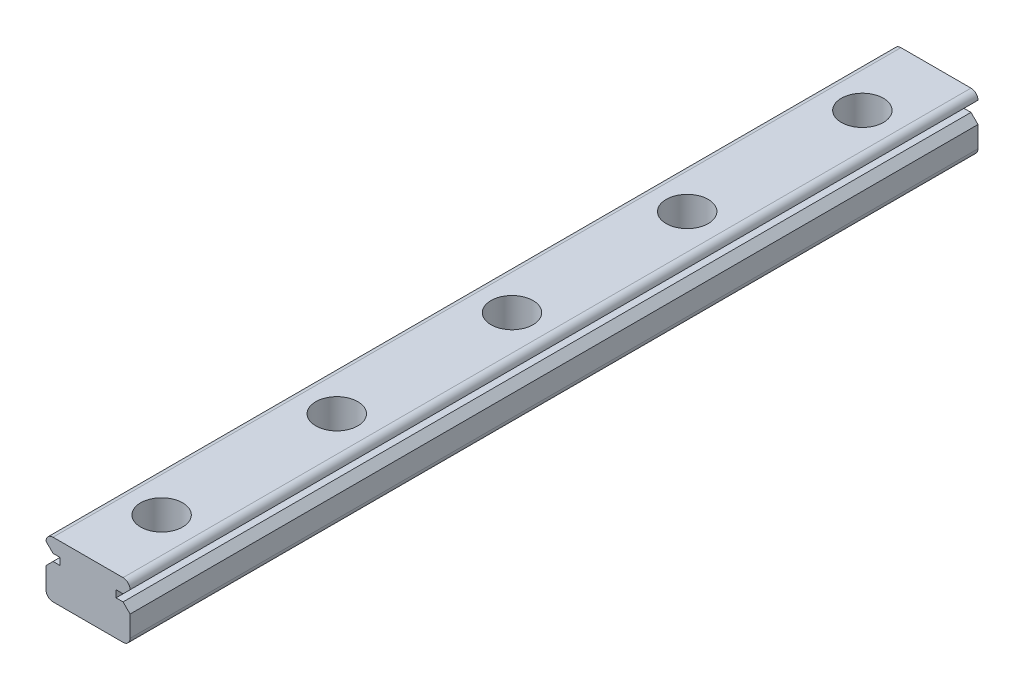
from build123d import *

# Parameters (mm, degrees)
BOSS_EXTRUDE1_DEPTH = 121
SKETCH2_R           = 3
CUT_EXTRUDE1_DEPTH  = 4.5
SKETCH3_R           = 1.75
CUT_EXTRUDE2_DEPTH  = 122.232215191


with BuildPart() as part:
    # Sketch1 → Boss-Extrude1 (new body)
    with BuildSketch(Plane.XY):
        with BuildLine():
            Line((-5, 4), (5, 4))
            ThreePointArc((5, 4), (5.707106781, 3.707106781), (6, 3))
            Line((6, 3), (5, 2))
            Line((5, 2), (4, 2))
            Line((4, 2), (4, 1))
            Line((4, 1), (5, 1))
            Line((5, 1), (6, 0))
            Line((6, 0), (6, -3))
            ThreePointArc((6, -3), (5.707106781, -3.707106781), (5, -4))
            Line((5, -4), (-5, -4))
            ThreePointArc((-5, -4), (-5.707106781, -3.707106781), (-6, -3))
            Line((-6, -3), (-6, 0))
            Line((-6, 0), (-5, 1))
            Line((-5, 1), (-4, 1))
            Line((-4, 1), (-4, 2))
            Line((-4, 2), (-5, 2))
            Line((-5, 2), (-6, 3))
            ThreePointArc((-6, 3), (-5.707106781, 3.707106781), (-5, 4))
        make_face()
    extrude(amount=BOSS_EXTRUDE1_DEPTH)

    # Sketch2 → Cut-Extrude1 (cut)
    with BuildSketch(Plane(origin=(0, 4, 0), x_dir=(1, 0, 0), z_dir=(0, 1, 0))):
        with Locations(Location((0, -10.5, 0), (0, 0, 270))):
            Circle(SKETCH2_R)
        with Locations(Location((0, -35.5, 0), (0, 0, 270))):
            Circle(SKETCH2_R)
        with Locations(Location((0, -60.5, 0), (0, 0, 270))):
            Circle(SKETCH2_R)
        with Locations(Location((0, -85.5, 0), (0, 0, 270))):
            Circle(SKETCH2_R)
        with Locations(Location((0, -110.5, 0), (0, 0, 270))):
            Circle(SKETCH2_R)
    extrude(amount=-CUT_EXTRUDE1_DEPTH, mode=Mode.SUBTRACT)

    # Sketch3 → Cut-Extrude2 (cut, through all)
    with BuildSketch(Plane(origin=(0, -0.5, 0), x_dir=(1, 0, 0), z_dir=(0, 1, 0))):
        with Locations(Location((0, -35.5, 0), (0, 0, 270))):
            Circle(SKETCH3_R)
        with Locations(Location((0, -10.5, 0), (0, 0, 270))):
            Circle(SKETCH3_R)
        with Locations(Location((0, -60.5, 0), (0, 0, 270))):
            Circle(SKETCH3_R)
        with Locations(Location((0, -85.5, 0), (0, 0, 270))):
            Circle(SKETCH3_R)
        with Locations(Location((0, -110.5, 0), (0, 0, 270))):
            Circle(SKETCH3_R)
    extrude(amount=-CUT_EXTRUDE2_DEPTH, mode=Mode.SUBTRACT)


solid = part.part
